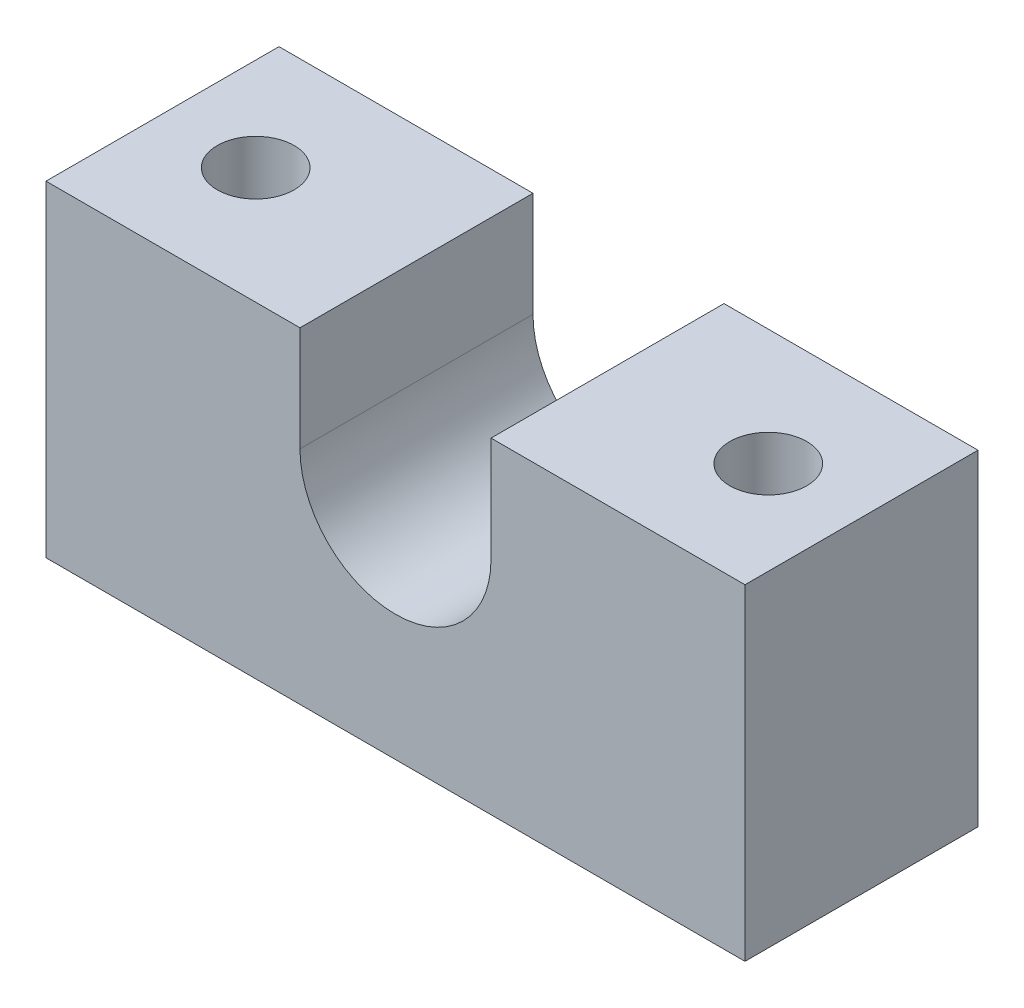
SolidWorks part; units mm, degrees
ref_plane "Front Plane" through (0, 0, 0) normal (0, 0, 1) x (1, 0, 0)
ref_plane "Top Plane" through (0, 0, 0) normal (0, 1, 0) x (1, 0, 0)
ref_plane "Right Plane" through (0, 0, 0) normal (1, 0, 0) x (0, 0, -1)
sketch "Sketch1" plane through (0, 0, 0) normal (0, 0, 1) x (1, 0, 0)
  line L1 (-15, 7) -> (15, 7)
  line L2 (-15, 7) -> (-15, -7)
  line L3 (-15, -7) -> (15, -7)
  line L4 (15, 7) -> (15, -7)
  line L5 (-15, 7) -> (15, -7) construction
  line L6 (-15, -7) -> (15, 7) construction
  point P0 (0, 0)
  dimension "D1" = 30
  dimension "D2" = 14
extrude "Boss-Extrude1" add sketch "Sketch1" along normal mid plane 10
sketch "Sketch2" plane through (0, 0, 5) normal (0, 0, 1) x (1, 0, 0)
  line L0 (0, 7) -> (0, 2.5) construction
  line L1 (15, 7) -> (-15, 7) construction
  line L2 (4.1, 7) -> (4.1, 2.5)
  line L3 (-4.1, 7) -> (-4.1, 2.5)
  arc A0 (4.1, 7) -> (-4.1, 7) centre (0, 7) ccw
  arc A1 (-4.1, 2.5) -> (4.1, 2.5) centre (0, 2.5) ccw
  point P5 (0, 4.75)
  dimension "D1" = 8.2
  dimension "D2" = 4.5
extrude "Cut-Extrude1" cut sketch "Sketch2" against normal through all
hole_wizard "M4 Tapped Hole1" positions "Sketch4" profile "Sketch3" tap size "M4" standard "Gb" end condition through all
sketch "Sketch4" plane through (0, 7, 0) normal (0, 1, 0) x (1, 0, 0)
  line L0 (0, 0) -> (0, 7.447) construction
  point P0 (-11, 0)
  point P2 (11, 0)
  dimension "D1" = 22
sketch "Sketch3" plane through (-11, 7, 0) normal (1, 0, 0) x (0, 0, 1)
  line L0 (0, 0) -> (0, 14)
  line L1 (0, 14) -> (1.65, 14)
  line L2 (1.65, 14) -> (1.65, 0)
  line L5 (1.65, 0) -> (0, 0)
  line L11 (0, -6.35) -> (0, 107.95) construction
  dimension "通孔螺纹孔钻头直径" = 3.3
  dimension "通孔螺纹孔钻头深度" = 14
cosmetic thread "Cosmetic Thread1"
cosmetic thread "Cosmetic Thread2"
